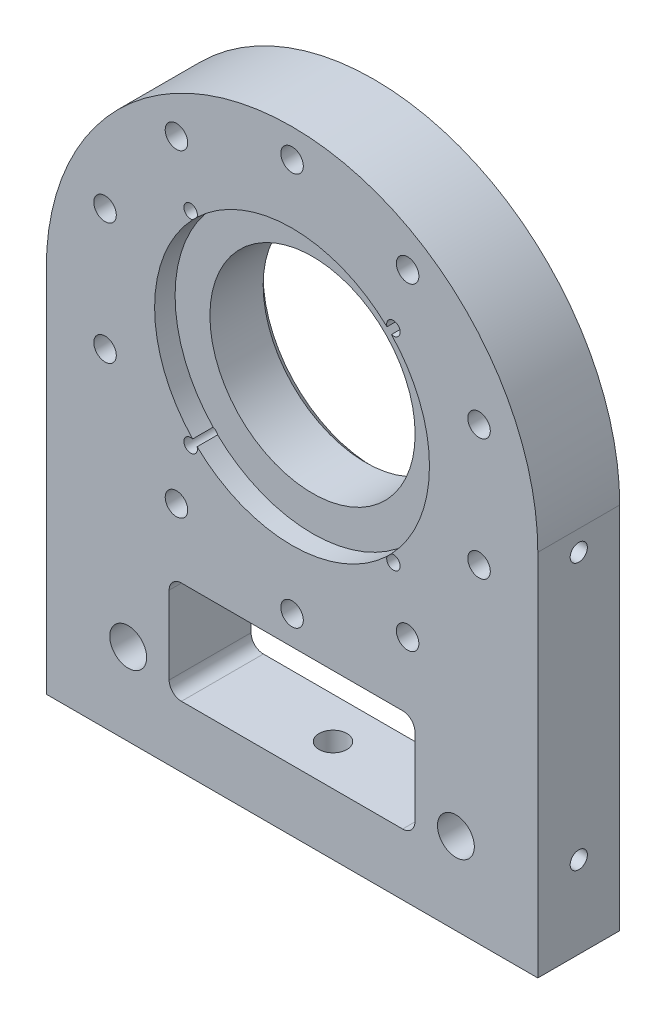
SolidWorks part; units mm, degrees
material "AL6061"
ref_plane "前视基准面" through (0, 0, 0) normal (0, 0, 1) x (1, 0, 0)
ref_plane "上视基准面" through (0, 0, 0) normal (0, 1, 0) x (1, 0, 0)
ref_plane "右视基准面" through (0, 0, 0) normal (1, 0, 0) x (0, 0, -1)
sketch "草图1" plane through (0, 0, 0) normal (0, 0, 1) x (1, 0, 0)
  line L0 (0, 73.4037) -> (0, -11.9326) construction
  line L3 (-60, 90) -> (-60, 0)
  line L4 (-60, 0) -> (60, 0)
  line L5 (60, 90) -> (60, 0)
  circle A1 centre (0, 95) radius 25.05
  arc A2 (-60, 90) -> (60, 90) centre (0, 90) cw
  dimension "D2" = 95
  dimension "D3" = 50.1
  dimension "D4" = 90
  dimension "D1" = 120
extrude "凸台-拉伸1" add sketch "草图1" along normal mid plane 20
hole_wizard "M8 螺纹孔1" positions "草图2" profile "草图3" tap size "M8" standard "GB"
sketch "草图2" plane through (0, 0, 0) normal (0, -1, 0) x (-1, 0, 0)
  line L0 (-54.3854, 0) -> (55.5026, 0) construction
  line L1 (0, 11.8825) -> (0, -11.8825) construction
  point P0 (50, 0)
  point P2 (0, 0)
  point P11 (-50, 0)
  dimension "D1" = 100
sketch "草图3" plane through (-50, 0, 0) normal (1, 0, 0) x (0, 0, -1)
  line L0 (0, 0) -> (0, 35.7929)
  line L1 (0, 35.7929) -> (3.4, 33.75)
  line L2 (3.4, 33.75) -> (3.4, 0)
  line L5 (3.4, 0) -> (0, 0)
  line L10 (0, 35.7929) -> (-3.4, 33.75) construction
  line L11 (0, -6.35) -> (0, 107.95) construction
  dimension "螺纹孔钻头直径" = 6.8
  dimension "螺纹孔钻头深度" = 33.75
  dimension "导头角度" = 118
cosmetic thread "孔螺蚊线1" parameters "D1"=30, "D2"=8
cosmetic thread "孔螺蚊线2" parameters "D1"=30, "D2"=8
cosmetic thread "孔螺蚊线3" parameters "D1"=30, "D2"=8
hole_wizard "Ø6.0 (6) 直径孔1" positions "草图4" profile "草图5" hole size "Ø6.0" standard "GB"
sketch "草图4" plane through (0, 0, 0) normal (0, -1, 0) x (-1, 0, 0)
  line L0 (-56.8228, 0) -> (54.8932, 0) construction
  line L1 (0, 11.3747) -> (0, -12.7966) construction
  point P0 (-35, 0)
  point P10 (35, 0)
  dimension "D1" = 70
sketch "草图5" plane through (35, 0, 0) normal (1, 0, 0) x (0, 0, -1)
  line L0 (0, 0) -> (0, 16.8026)
  line L1 (0, 16.8026) -> (3, 15)
  line L2 (3, 15) -> (3, 0)
  line L5 (3, 0) -> (0, 0)
  line L10 (0, 16.8026) -> (-3, 15) construction
  line L11 (0, -6.35) -> (0, 107.95) construction
  dimension "孔直径" = 6
  dimension "孔深度" = 15
  dimension "导头角度" = 118
sketch "草图6" plane through (0, 0, 10) normal (0, 0, 1) x (1, 0, 0)
  circle A0 centre (0, 95) radius 33.55
  dimension "D1" = 67.1
extrude "切除-拉伸1" cut sketch "草图6" against normal blind 5
hole_wizard "M4 螺纹孔1" positions "草图7" profile "草图8" tap size "M4" standard "GB" end condition through all
sketch "草图7" plane through (0, 0, -10) normal (0, 0, -1) x (-1, 0, 0)
  line L0 (0, 256.6299) -> (0, -8.0004) construction
  line L1 (0, 95) -> (-71.4339, 95) construction
  line L2 (0, 95) -> (-97.8899, 192.8899) construction
  circle A0 centre (0, 95) radius 35 construction
  point P0 (-24.7487, 119.7487)
  dimension "D2" = 70
  dimension "D1" = 45
sketch "草图8" plane through (24.7487, 119.7487, -10) normal (1, 0, 0) x (0, 1, 0)
  line L0 (0, 0) -> (0, 20)
  line L1 (0, 20) -> (1.65, 20)
  line L2 (1.65, 20) -> (1.65, 0)
  line L5 (1.65, 0) -> (0, 0)
  line L11 (0, -6.35) -> (0, 107.95) construction
  dimension "通孔螺纹孔钻头直径" = 3.3
  dimension "通孔螺纹孔钻头深度" = 20
cosmetic thread "孔螺蚊线4" parameters "D2"=4
pattern_circular "阵列(圆周)1" count 4 over 360 about axis through (0, 95, 0) along (0, 0, 1) of "M4 螺纹孔1"
chamfer "倒角1" distance 2 angle 45 1 edges at (25.05, 95, -10)
hole_wizard "打孔尺寸(%根据)内六角圆柱头螺钉的类型2" positions "草图9" profile "草图10" counterbore size "M5" standard "GB" end condition through all
sketch "草图9" plane through (0, 0, -10) normal (0, 0, -1) x (-1, 0, 0)
  line L0 (0, 257.9287) -> (0, -5.7275) construction
  line L1 (0, 95) -> (-61.3683, 95) construction
  circle A0 centre (0, 95) radius 48 construction
  point P0 (0, 143)
  dimension "D1" = 96
sketch "草图10" plane through (0, 143, -10) normal (1, 0, 0) x (0, 1, 0)
  line L0 (0, 0) -> (0, 20)
  line L1 (0, 20) -> (2.75, 20)
  line L3 (2.75, 20) -> (2.75, 5.7)
  line L4 (2.75, 5.7) -> (5, 5.7)
  line L5 (5, 5.7) -> (5, 0)
  line L7 (5, 0) -> (0, 0)
  line L11 (0, -6.35) -> (0, 107.95) construction
  dimension "通孔孔直径" = 5.5
  dimension "通孔孔深度" = 20
  dimension "柱形沉头孔直径" = 10
  dimension "柱形沉头孔深度" = 5.7
pattern_circular "阵列(圆周)2" count 10 over 360 about axis through (0, 95, 0) along (0, 0, 1) of "打孔尺寸(%根据)内六角圆柱头螺钉的类型2"
hole_wizard "打孔尺寸(%根据)内六角圆柱头螺钉的类型2" positions "草图11" profile "草图12" counterbore size "M8" standard "GB" end condition through all
sketch "草图11" plane through (0, 0, -10) normal (0, 0, -1) x (-1, 0, 0)
  line L0 (0, 95) -> (0, -8.5412) construction
  line L1 (60, 0) -> (-60, 0) construction
  point P0 (-40, 20)
  point P8 (40, 20)
  dimension "D1" = 80
  dimension "D2" = 20
sketch "草图12" plane through (40, 20, -10) normal (1, 0, 0) x (0, 1, 0)
  line L0 (0, 0) -> (0, 20)
  line L1 (0, 20) -> (4.5, 20)
  line L3 (4.5, 20) -> (4.5, 9)
  line L4 (4.5, 9) -> (7.5, 9)
  line L5 (7.5, 9) -> (7.5, 0)
  line L7 (7.5, 0) -> (0, 0)
  line L11 (0, -6.35) -> (0, 107.95) construction
  dimension "通孔孔直径" = 9
  dimension "通孔孔深度" = 20
  dimension "柱形沉头孔直径" = 15
  dimension "柱形沉头孔深度" = 9
sketch "草图13" plane through (0, 0, -10) normal (0, 0, -1) x (-1, 0, 0)
  line L0 (0, 157.5093) -> (0, -4.6932) construction
  line L1 (60, 0) -> (-60, 0) construction
  line L2 (-27, 40) -> (27, 40)
  line L3 (-30, 37) -> (-30, 18)
  line L4 (-27, 15) -> (27, 15)
  line L5 (30, 37) -> (30, 18)
  arc A0 (-30, 18) -> (-27, 15) centre (-27, 18) ccw
  arc A1 (27, 40) -> (30, 37) centre (27, 37) cw
  arc A2 (27, 15) -> (30, 18) centre (27, 18) ccw
  arc A3 (-27, 40) -> (-30, 37) centre (-27, 37) ccw
  dimension "D1" = 3
  dimension "D2" = 60
  dimension "D3" = 25
  dimension "D4" = 15
extrude "切除-拉伸2" cut sketch "草图13" against normal through all
hole_wizard "M5 螺纹孔1" positions "草图14" profile "草图15" tap size "M5" standard "ISO"
sketch "草图14" plane through (60, 0, 0) normal (1, 0, 0) x (0, 0, -1)
  line L0 (0, -5.0903) -> (0, 140.8325) construction
  line L1 (-10, 0) -> (10, 0) construction
  point P0 (0, 20)
  point P2 (0, 85)
  dimension "D1" = 20
  dimension "D2" = 65
sketch "草图15" plane through (60, 20, 0) normal (0, 1, 0) x (0, 0, -1)
  line L0 (0, 0) -> (0, 15.6618)
  line L1 (0, 15.6618) -> (2.1, 14.4)
  line L2 (2.1, 14.4) -> (2.1, 0)
  line L5 (2.1, 0) -> (0, 0)
  line L10 (0, 15.6618) -> (-2.1, 14.4) construction
  line L11 (0, -6.35) -> (0, 107.95) construction
  dimension "螺纹孔钻头直径" = 4.2
  dimension "螺纹孔钻头深度" = 14.4
  dimension "导头角度" = 118
cosmetic thread "孔螺蚊线5" parameters "D1"=12, "D2"=5
cosmetic thread "孔螺蚊线6" parameters "D1"=12, "D2"=5
mirror "镜向1" about plane through (0, 0, 0) normal (1, 0, 0) of "M5 螺纹孔1"
